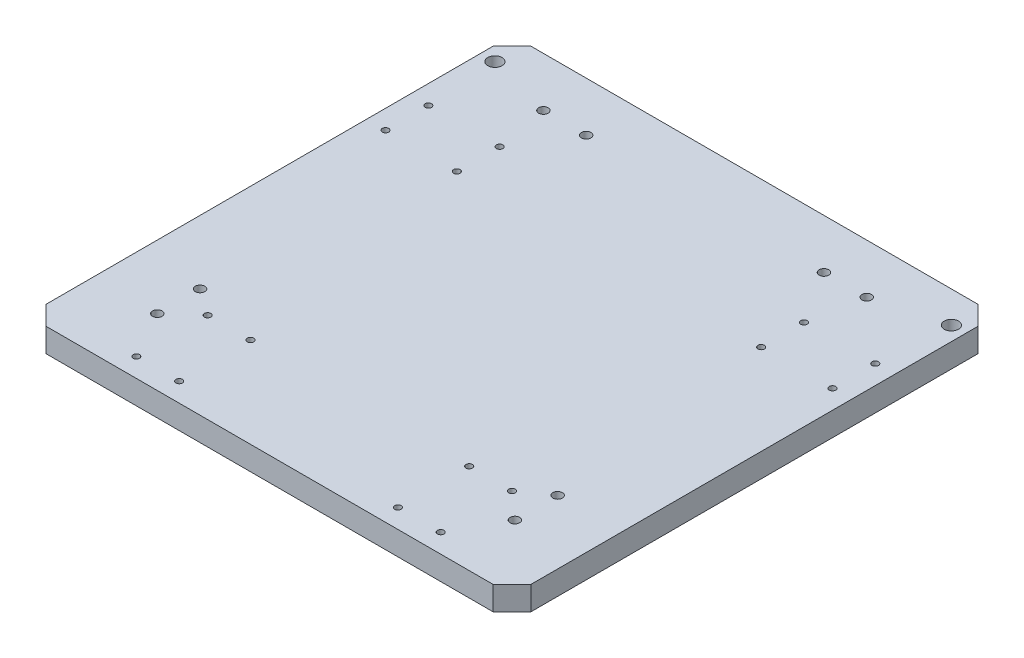
SolidWorks part; units mm, degrees
material "S45C"
ref_plane "前视基准面" through (0, 0, 0) normal (0, 0, 1) x (1, 0, 0)
ref_plane "上视基准面" through (0, 0, 0) normal (0, 1, 0) x (1, 0, 0)
ref_plane "右视基准面" through (0, 0, 0) normal (1, 0, 0) x (0, 0, -1)
sketch "草图1" plane through (0, 0, 0) normal (0, 1, 0) x (1, 0, 0)
  line L1 (255, -255) -> (-255, -255)
  line L2 (255, -255) -> (255, 255)
  line L3 (255, 255) -> (-255, 255)
  line L4 (-255, -255) -> (-255, 255)
  line L5 (255, -255) -> (-255, 255) construction
  line L6 (255, 255) -> (-255, -255) construction
  point P0 (0, 0)
  dimension "D1" = 510
  dimension "D2" = 510
extrude "凸台-拉伸1" add sketch "草图1" along normal mid plane 25
hole_wizard "Ø2.0 (2) 直径孔1" positions "草图2" profile "草图3" hole size "Ø2.0" standard "ISO"
sketch "草图2" plane through (0, 12.5, 0) normal (0, 1, 0) x (1, 0, 0)
  point P0 (-193.5183, 176.3987)
  point P3 (-237.2222, 165.6762)
  point P6 (-254.8548, 237.5447)
  point P9 (-211.1509, 248.2672)
  point P12 (75.3522, 318.5592)
  point P15 (92.9848, 246.6906)
  point P18 (49.2809, 235.9681)
  point P21 (31.6484, 307.8367)
  point P24 (264.0642, -64.5085)
  point P27 (274.7867, -108.2123)
  point P30 (202.9181, -125.8449)
  point P33 (192.1956, -82.141)
  point P44 (-244.8431, -189.366)
  point P47 (-234.1206, -233.0698)
  point P55 (-162.252, -215.4373)
  point P58 (-172.9745, -171.7334)
sketch "草图3" plane through (-193.5183, 12.5, -176.3987) normal (1, 0, 0) x (0, 0, 1)
  line L0 (0, 0) -> (0, 25)
  line L1 (0, 25) -> (1, 25)
  line L2 (1, 25) -> (1, 0)
  line L5 (1, 0) -> (0, 0)
  line L11 (0, -6.35) -> (0, 107.95) construction
  dimension "通孔孔直径" = 2
  dimension "通孔孔深度" = 25
hole_wizard "Ø10.0 (10) 直径孔2" positions "草图4" profile "草图5" hole size "Ø10.0" standard "GB" end condition through all
sketch "草图4" plane through (0, -12.5, 0) normal (0, -1, 0) x (-1, 0, 0)
  line L0 (255, 255) -> (255, -255) construction
  line L1 (-255, 255) -> (255, 255) construction
  point P3 (188, -185)
  point P6 (188, -140)
  point P12 (-188, -185)
  point P18 (-188, -140)
  point P24 (170, 203)
  point P27 (125, 203)
  point P36 (-125, 203)
  point P39 (-170, 203)
  dimension "D1" = 67
  dimension "D2" = 376
  dimension "D3" = 45
  dimension "D4" = 395
  dimension "D5" = 45
  dimension "D6" = 250
  dimension "D7" = 45
  dimension "D8" = 52
  dimension "D9" = 85
sketch "草图5" plane through (-188, -12.5, 185) normal (1, 0, 0) x (0, 0, -1)
  line L0 (0, 0) -> (0, 25)
  line L1 (0, 25) -> (5, 25)
  line L2 (5, 25) -> (5, 0)
  line L5 (5, 0) -> (0, 0)
  line L11 (0, -6.35) -> (0, 107.95) construction
  dimension "通孔孔直径" = 10
  dimension "通孔孔深度" = 25
hole_wizard "Ø15.0 (15) 直径孔1" positions "草图6" profile "草图7" hole size "Ø15.0" standard "GB" end condition through all
sketch "草图6" plane through (0, 12.5, 0) normal (0, 1, 0) x (1, 0, 0)
  line L0 (-255, 255) -> (-255, -255) construction
  line L1 (255, 255) -> (-255, 255) construction
  point P0 (-240, -334.5687)
  point P3 (-240, 222)
  point P6 (240, 222)
  point P9 (240, -307.6472)
  dimension "D1" = 480
  dimension "D2" = 15
  dimension "D3" = 33
sketch "草图7" plane through (-240, 12.5, 334.5687) normal (1, 0, 0) x (0, 0, 1)
  line L0 (0, 0) -> (0, 25)
  line L1 (0, 25) -> (7.5, 25)
  line L2 (7.5, 25) -> (7.5, 0)
  line L5 (7.5, 0) -> (0, 0)
  line L11 (0, -6.35) -> (0, 107.95) construction
  dimension "通孔孔直径" = 15
  dimension "通孔孔深度" = 25
hole_wizard "M8 螺纹孔1" positions "草图8" profile "草图9" tap size "M8" standard "GB" end condition through all
sketch "草图8" plane through (0, -12.5, 0) normal (0, -1, 0) x (-1, 0, 0)
  line L0 (0, 255) -> (0, -335.0058) construction
  line L1 (-255, 255) -> (255, 255) construction
  line L4 (115, -160) -> (160, -160) construction
  line L5 (115, -160) -> (115, -235) construction
  line L6 (115, -235) -> (160, -235) construction
  line L7 (160, -160) -> (160, -235) construction
  line L8 (255, -255) -> (-255, -255) construction
  line L10 (-160, -160) -> (-115, -160) construction
  line L11 (-160, -160) -> (-160, -235) construction
  line L12 (-160, -235) -> (-115, -235) construction
  line L13 (-115, -160) -> (-115, -235) construction
  line L15 (160, 147) -> (235, 147) construction
  line L16 (160, 147) -> (160, 102) construction
  line L17 (160, 102) -> (235, 102) construction
  line L18 (235, 147) -> (235, 102) construction
  line L20 (-235, 147) -> (-160, 147) construction
  line L21 (-235, 147) -> (-235, 102) construction
  line L22 (-235, 102) -> (-160, 102) construction
  line L23 (-160, 147) -> (-160, 102) construction
  line L24 (255, 255) -> (255, -255) construction
  line L25 (-255, -255) -> (-255, 255) construction
  line L27 (255, 255) -> (255, -255) construction
  line L28 (-255, 255) -> (255, 255) construction
  point P0 (115, -160)
  point P2 (160, -160)
  point P4 (115, -235)
  point P6 (160, -235)
  point P8 (-160, -160)
  point P10 (-115, -160)
  point P12 (-115, -235)
  point P14 (-160, -235)
  point P16 (-235, 147)
  point P18 (-160, 147)
  point P20 (-160, 102)
  point P22 (-235, 102)
  point P24 (160, 147)
  point P26 (235, 147)
  point P28 (235, 102)
  point P30 (160, 102)
  point P152 (137.5, -235)
  dimension "D3" = 45
  dimension "D9" = 95
  dimension "D15" = 108
  dimension "D2" = 20
  dimension "D4" = 75
  dimension "D5" = 230
  dimension "D6" = 45
  dimension "D7" = 75
  dimension "D8" = 20
  dimension "D10" = 45
  dimension "D11" = 75
  dimension "D12" = 20
  dimension "D13" = 75
  dimension "D14" = 45
  dimension "D16" = 20
sketch "草图9" plane through (-115, -12.5, 160) normal (1, 0, 0) x (0, 0, -1)
  line L0 (0, 0) -> (0, 25)
  line L1 (0, 25) -> (3.4, 25)
  line L2 (3.4, 25) -> (3.4, 0)
  line L5 (3.4, 0) -> (0, 0)
  line L11 (0, -6.35) -> (0, 107.95) construction
  dimension "通孔螺纹孔钻头直径" = 6.8
  dimension "通孔螺纹孔钻头深度" = 25
cosmetic thread "孔螺蚊线1" parameters "D1"=25, "D2"=8
cosmetic thread "孔螺蚊线2" parameters "D1"=25, "D2"=8
cosmetic thread "孔螺蚊线3" parameters "D1"=25, "D2"=8
cosmetic thread "孔螺蚊线4" parameters "D1"=25, "D2"=8
cosmetic thread "孔螺蚊线5" parameters "D1"=25, "D2"=8
cosmetic thread "孔螺蚊线6" parameters "D1"=25, "D2"=8
cosmetic thread "孔螺蚊线7" parameters "D1"=25, "D2"=8
cosmetic thread "孔螺蚊线8" parameters "D1"=25, "D2"=8
cosmetic thread "孔螺蚊线9" parameters "D1"=25, "D2"=8
cosmetic thread "孔螺蚊线10" parameters "D1"=25, "D2"=8
cosmetic thread "孔螺蚊线11" parameters "D1"=25, "D2"=8
cosmetic thread "孔螺蚊线12" parameters "D1"=25, "D2"=8
cosmetic thread "孔螺蚊线13" parameters "D1"=25, "D2"=8
cosmetic thread "孔螺蚊线14" parameters "D1"=25, "D2"=8
cosmetic thread "孔螺蚊线15" parameters "D1"=25, "D2"=8
cosmetic thread "孔螺蚊线16" parameters "D1"=25, "D2"=8
chamfer "倒角1" distance 20 angle 45 4 edges at (255, 0, -255) (-255, 0, -255) (-255, 0, 255) (255, 0, 255)
